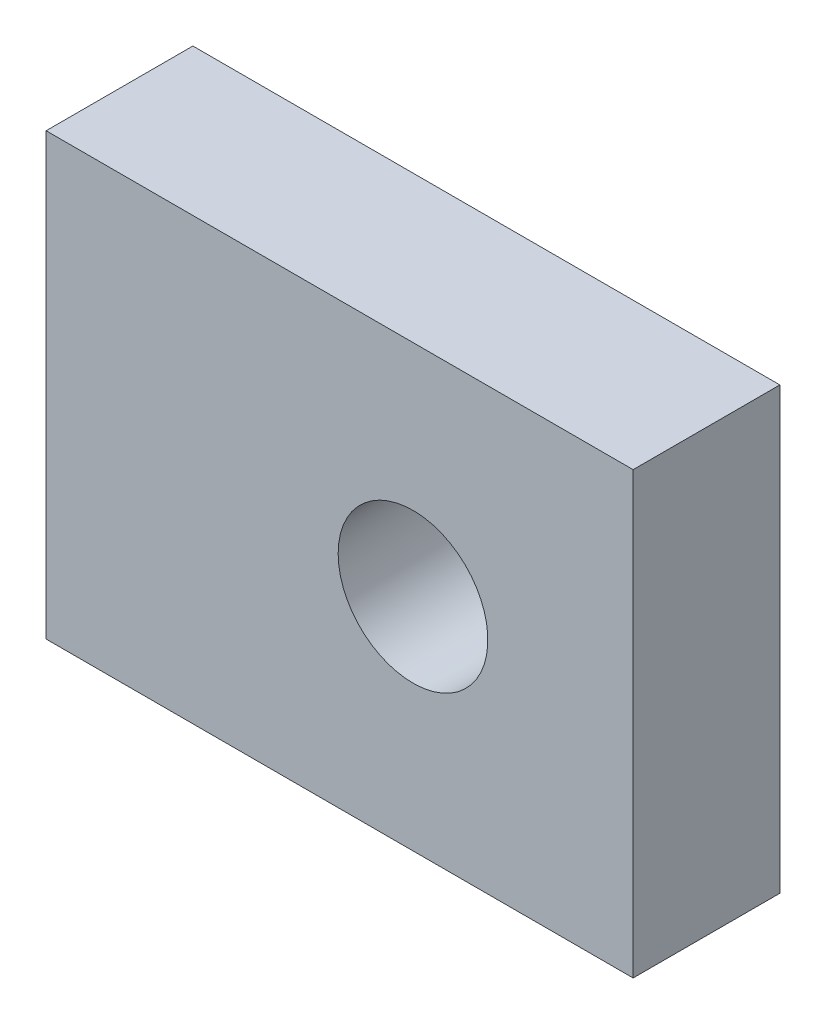
from build123d import *

# Parameters (mm, degrees)
SKETCH1_W           = 40
SKETCH1_H           = 30
SKETCH1_R           = 5
BOSS_EXTRUDE1_DEPTH = 10
M12_TAPPED_HOLE1_D  = 10.2


with BuildPart() as part:
    # Sketch1 → Boss-Extrude1 (new body)
    with BuildSketch(Plane.XY):
        Rectangle(SKETCH1_W, SKETCH1_H)
        with Locations((5, 0)):
            Circle(SKETCH1_R, mode=Mode.SUBTRACT)
    extrude(amount=BOSS_EXTRUDE1_DEPTH)

    # M12 Tapped Hole1 (through all)
    with Locations(Plane(origin=(5, 0, 0), x_dir=(-1, 0, 0), z_dir=(0, 0, -1))):
        with Locations((0, 0)):
            Hole(M12_TAPPED_HOLE1_D / 2)


solid = part.part
